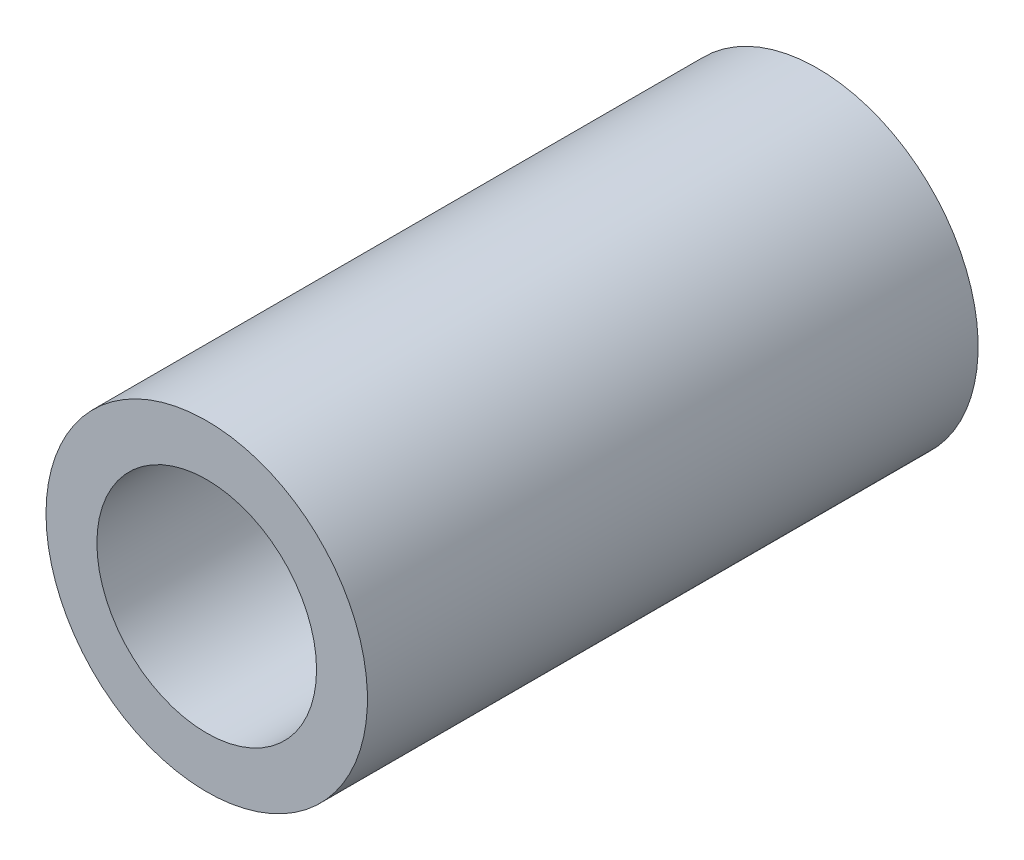
SolidWorks part; units mm, degrees
ref_plane "前视基准面" through (0, 0, 0) normal (0, 0, 1) x (1, 0, 0)
ref_plane "上视基准面" through (0, 0, 0) normal (0, 1, 0) x (1, 0, 0)
ref_plane "右视基准面" through (0, 0, 0) normal (1, 0, 0) x (0, 0, -1)
sketch "草图1" plane through (0, 0, 0) normal (0, 0, 1) x (1, 0, 0)
  circle A0 centre (0, 0) radius 15
  circle A1 centre (0, 0) radius 10.25
  dimension "D1" = 20.5
  dimension "D2" = 30
extrude "凸台-拉伸1" add sketch "草图1" along normal mid plane 57
chamfer "倒角1" [suppressed] distance 1 angle 45
